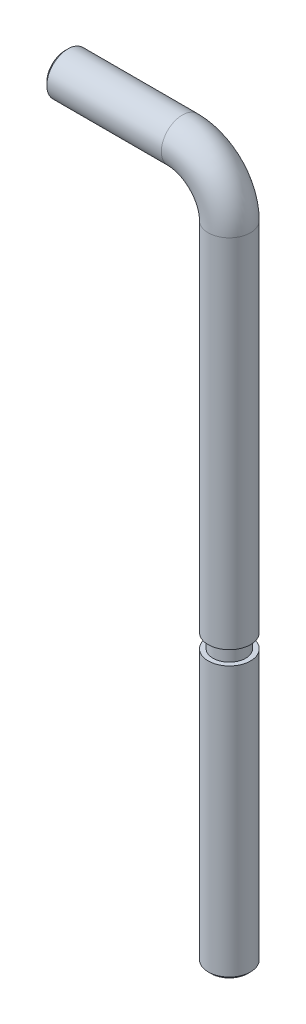
SolidWorks part; units mm, degrees
material "不锈钢 (铁素体)"
ref_plane "Front Plane" through (0, 0, 0) normal (0, 0, 1) x (1, 0, 0)
ref_plane "Top Plane" through (0, 0, 0) normal (0, 1, 0) x (1, 0, 0)
ref_plane "Right Plane" through (0, 0, 0) normal (1, 0, 0) x (0, 0, -1)
sketch "Sketch1" plane through (0, 0, 0) normal (0, 0, 1) x (1, 0, 0)
  line L0 (0, 0) -> (0, 68.5)
  line L1 (-5, 73.5) -> (-17.5, 73.5)
  arc A0 (0, 68.5) -> (-5, 73.5) centre (-5, 68.5) ccw
  point P6 (0, 73.5)
  dimension "D3" = 5
  dimension "D1" = 73.5
  dimension "D2" = 17.5
sketch "Sketch2" plane through (0, 0, 0) normal (0, 1, 0) x (1, 0, 0)
  circle A0 centre (0, 0) radius 2.25
  dimension "D1" = 4.5
sweep "Sweep1" add profiles "Sketch2" path "Sketch1"
sketch "Sketch3" plane through (0, 0, 0) normal (1, 0, 0) x (0, 0, -1)
  line L0 (2.25, 0) -> (2.25, 68.5) construction
  line L1 (1.75, 29) -> (2.25, 29)
  line L2 (1.75, 29) -> (1.75, 30.5)
  line L3 (1.75, 30.5) -> (2.25, 30.5)
  line L4 (2.25, 29) -> (2.25, 30.5)
  line L5 (1.75, 29) -> (2.25, 30.5) construction
  line L6 (1.75, 30.5) -> (2.25, 29) construction
  line L7 (0, 0) -> (0, 51.3602) construction
  point P0 (2, 29.75)
  dimension "D1" = 0.5
  dimension "D2" = 1.5
  dimension "D3" = 29
revolve "Cut-Revolve1" cut sketch "Sketch3" angle 360 about L7
chamfer "Chamfer1" distance 0.3 angle 45 2 edges at (-17.5, 73.5, 2.25) (0, 0, 2.25)
